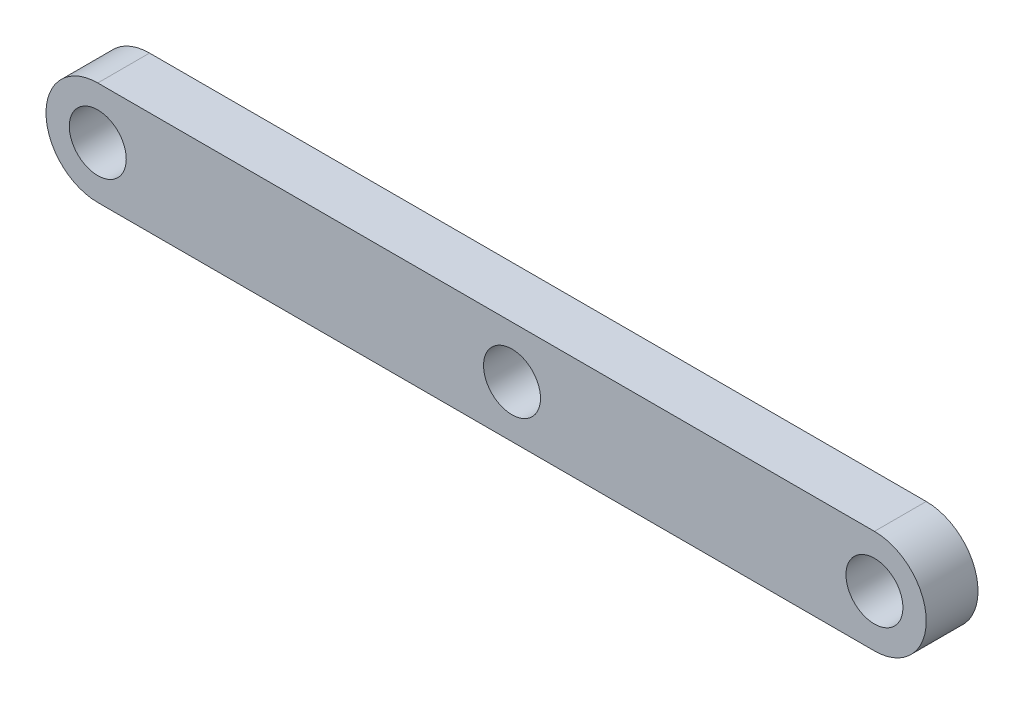
SolidWorks part; units mm, degrees
ref_plane "Alzado" through (0, 0, 0) normal (0, 0, 1) x (1, 0, 0)
ref_plane "Planta" through (0, 0, 0) normal (0, 1, 0) x (1, 0, 0)
ref_plane "Vista lateral" through (0, 0, 0) normal (1, 0, 0) x (0, 0, -1)
sketch "Sketch1" plane through (0, 0, 0) normal (0, 0, 1) x (1, 0, 0)
  line L0 (-7.5, 0) -> (7.5, 0) construction
  line L1 (-7.5, 1) -> (7.5, 1)
  line L2 (-7.5, -1) -> (7.5, -1)
  arc A0 (-7.5, 1) -> (-7.5, -1) centre (-7.5, 0) ccw
  arc A1 (7.5, -1) -> (7.5, 1) centre (7.5, 0) ccw
  circle A2 centre (-7.5, 0) radius 0.55
  circle A3 centre (7.5, 0) radius 0.55
  circle A4 centre (0.5, 0) radius 0.55
  point P3 (0, 0)
  dimension "D3" = 1.1
  dimension "D4" = 8
  dimension "D1" = 15
  dimension "D2" = 2
extrude "Thigh1 length" add sketch "Sketch1" along normal mid plane 1
sketch "Sketch2" plane through (0, 0, 0.5) normal (0, 0, 1) x (1, 0, 0)
  circle A0 centre (-7.5, 0) radius 1.8
  circle A1 centre (7.5, 0) radius 1.8
  circle A2 centre (0.5, 0) radius 1.8
  dimension "D1" = 3.6
extrude "Cortar-Extruir1" [suppressed] cut sketch "Sketch2" against normal blind 1
